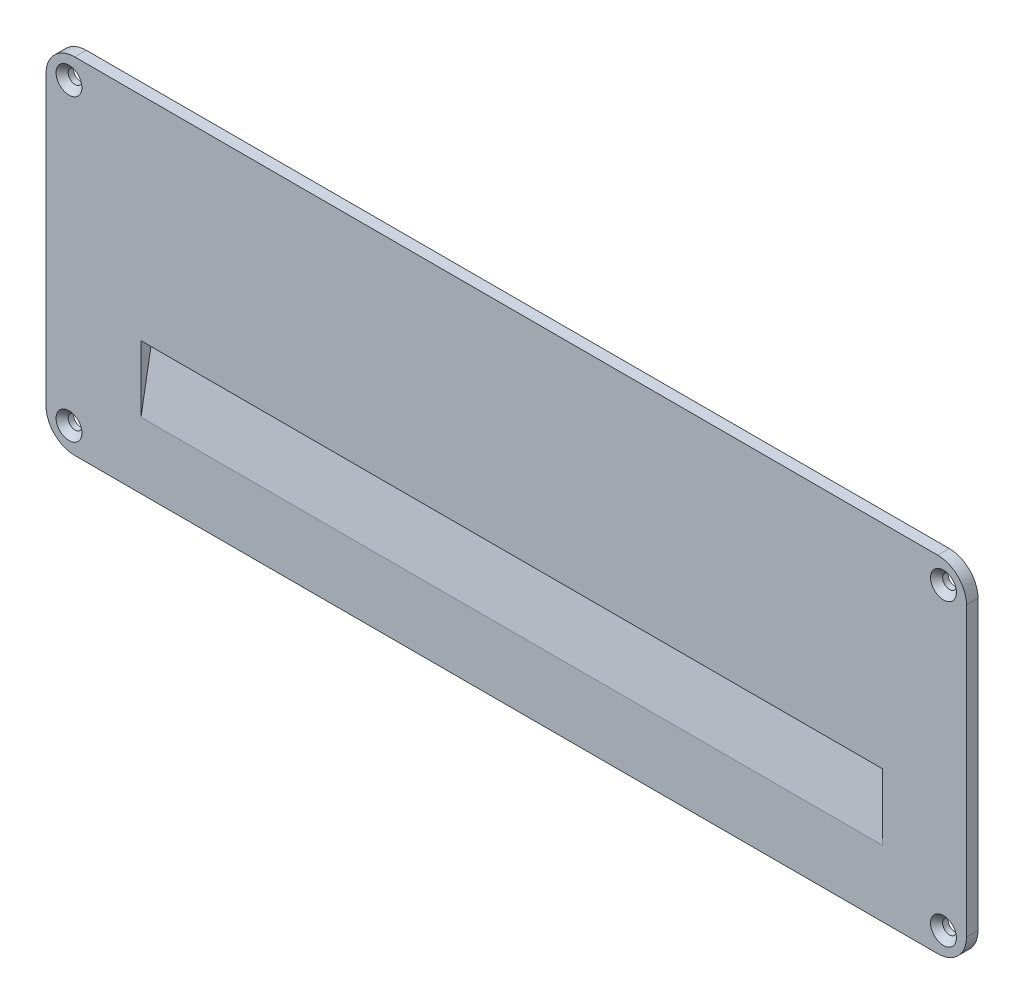
SolidWorks part; units mm, degrees
material "AISI 304"
ref_plane "Front Plane" through (0, 0, 0) normal (0, 0, 1) x (1, 0, 0)
ref_plane "Top Plane" through (0, 0, 0) normal (0, 1, 0) x (1, 0, 0)
ref_plane "Right Plane" through (0, 0, 0) normal (1, 0, 0) x (0, 0, -1)
sketch "Sketch1" plane through (0, 0, 0) normal (0, 0, 1) x (1, 0, 0)
  line L1 (-80, -30) -> (80, -30)
  line L2 (-80, -30) -> (-80, 30)
  line L3 (-80, 30) -> (80, 30)
  line L4 (80, -30) -> (80, 30)
  line L5 (-80, -30) -> (80, 30) construction
  line L6 (-80, 30) -> (80, -30) construction
  point P0 (0, 0)
  dimension "D1" = 160
  dimension "D2" = 60
extrude "Boss-Extrude1" add sketch "Sketch1" along normal blind 2
sketch "Sketch2" plane through (0, 0, 2) normal (0, 0, 1) x (1, 0, 0)
  line L0 (0, 0) -> (0, 57.8431) construction
  line L1 (0, 0) -> (-105.9748, 0) construction
  line L2 (-80, 30) -> (-80, -30) construction
  line L3 (80, 30) -> (-80, 30) construction
  circle A0 centre (-76, 26) radius 0.5
  circle A1 centre (76, 26) radius 0.5
  circle A2 centre (76, -26) radius 0.5
  circle A3 centre (-76, -26) radius 0.5
  dimension "D1" = 1
  dimension "D2" = 4
  dimension "D3" = 4
extrude "Cut-Extrude1" cut sketch "Sketch2" against normal blind 2
hole_wizard "Pilot hole size (% per cross) slotted countersunk wood screw type1" positions "Sketch3" profile "Sketch4" countersink size "M2" standard "GB"
sketch "Sketch3" plane through (0, 0, 2) normal (0, 0, 1) x (1, 0, 0)
  point P0 (-76, 26)
  point P3 (76, 26)
  point P6 (76, -26)
  point P9 (-76, -26)
sketch "Sketch4" plane through (-76, 26, 2) normal (1, 0, 0) x (0, -1, 0)
  line L0 (0, 0) -> (0, 8.221)
  line L1 (0, 8.221) -> (1.2, 7.5)
  line L2 (1.2, 7.5) -> (1.2, 1.05)
  line L3 (1.2, 1.05) -> (2.25, 0)
  line L5 (2.25, 0) -> (0, 0)
  line L6 (-1.2, 1.05) -> (-2.25, 0) construction
  line L10 (0, 8.221) -> (-1.2, 7.5) construction
  line L11 (0, -6.35) -> (0, 107.95) construction
  dimension "孔直径" = 2.4
  dimension "孔深度" = 7.5
  dimension "近端锥形沉头孔直径" = 4.5
  dimension "近端锥形沉头孔角度" = 90
  dimension "导头角度" = 118
ref_plane "Plane2" through (0, -29.4374, 5.1906) normal (0, -0.9848, 0.1736) x (1, 0, 0)
sketch "Sketch6" plane through (0, -29.4374, 5.1906) normal (0, -0.9848, 0.1736) x (1, 0, 0)
  line L1 (-63.4872, 0.7612) -> (65.4294, 0.7612)
  line L2 (-63.4872, 0.7612) -> (-63.4872, -1.2388)
  line L3 (-63.4872, -1.2388) -> (65.4294, -1.2388)
  line L4 (65.4294, 0.7612) -> (65.4294, -1.2388)
  dimension "D1" = 2
extrude "Cut-Extrude3" cut sketch "Sketch6" against normal blind 100
fillet "Fillet1" radius 5 4 edges at (80, -30, 1) (-80, -30, 1) (80, 30, 1) (-80, 30, 1)
